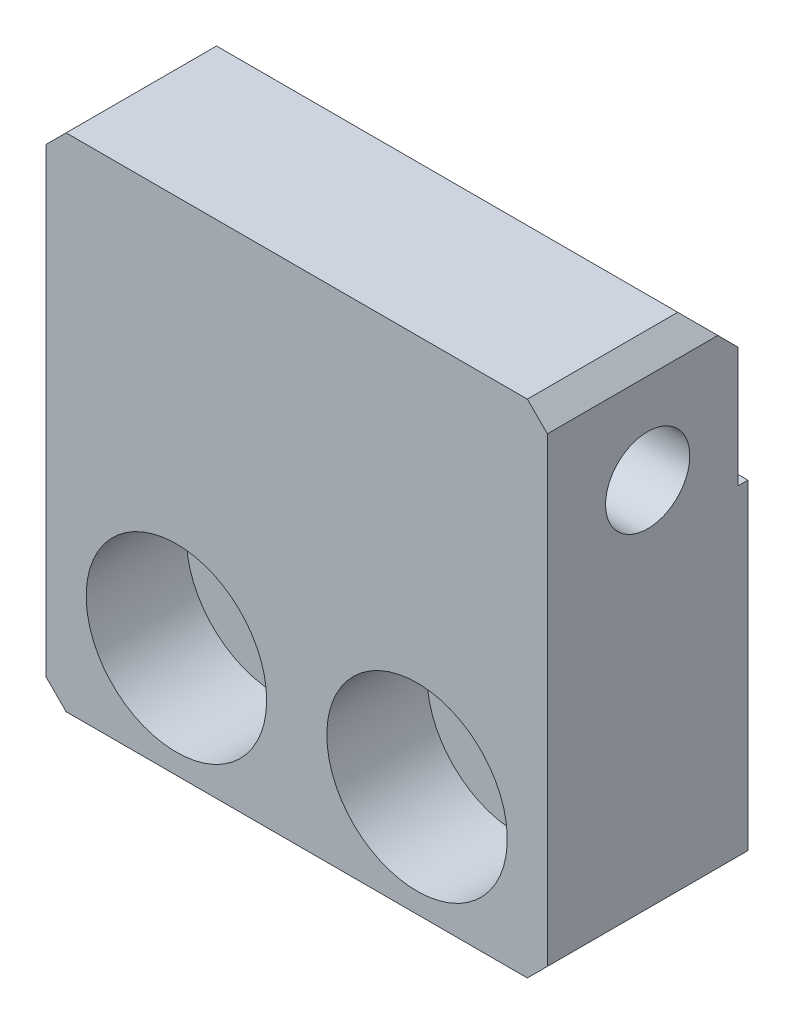
from build123d import *

# Parameters (mm, degrees)
SKETCH1_W           = 25
SKETCH1_H           = 25
BOSS_EXTRUDE1_DEPTH = 10
SKETCH3_R           = 4.5
CUT_EXTRUDE2_DEPTH  = 5
SKETCH4_R           = 2.25
CUT_EXTRUDE3_DEPTH  = 14
SKETCH5_R           = 0.905939467
CUT_EXTRUDE4_DEPTH  = 31
M5_TAPPED_HOLE1_D   = 4.2
CHAMFER1_SIZE       = 1
SKETCH8_W           = 0.5
SKETCH8_H           = 8
CUT_EXTRUDE5_DEPTH  = 31
CHAMFER2_SIZE       = 2


with BuildPart() as part:
    # Sketch1 → Boss-Extrude1 (new body)
    with BuildSketch(Plane.XY):
        Rectangle(SKETCH1_W, SKETCH1_H)
    extrude(amount=BOSS_EXTRUDE1_DEPTH)

    # Sketch3 → Cut-Extrude2 (cut)
    with BuildSketch(Plane.XY.offset(10)):
        with Locations((-6, -7)):
            Circle(SKETCH3_R)
        with Locations(Location((6, -7, 0), (0, 0, 180))):
            Circle(SKETCH3_R)
    extrude(amount=-CUT_EXTRUDE2_DEPTH, mode=Mode.SUBTRACT)

    # Sketch4 → Cut-Extrude3 (cut)
    with BuildSketch(Plane.XY.offset(10)):
        with Locations((-6, -7)):
            Circle(SKETCH4_R)
        with Locations((6, -7)):
            Circle(SKETCH4_R)
    extrude(amount=-CUT_EXTRUDE3_DEPTH, mode=Mode.SUBTRACT)

    # Sketch5 → Cut-Extrude4 (cut)
    with BuildSketch(Plane.ZY.offset(12.5)):
        with Locations(Location((5, 7, 0), (0, 0, 270))):
            Circle(SKETCH5_R)
    extrude(amount=-CUT_EXTRUDE4_DEPTH, mode=Mode.SUBTRACT)

    # M5 Tapped Hole1 (through all)
    with Locations(Plane(origin=(-12.5, 7, 5), x_dir=(0, -1, 0), z_dir=(-1, 0, 0))):
        with Locations((0, 0)):
            Hole(M5_TAPPED_HOLE1_D / 2)

    # Chamfer1
    chamfer1_edges = [part.edges().sort_by_distance(p)[0] for p in [
        (12.5, -12.5, 5),
        (-12.5, -12.5, 5),
        (-12.5, 12.5, 5),
        (12.5, 12.5, 5),
    ]]
    chamfer(chamfer1_edges, length=CHAMFER1_SIZE)

    # Sketch8 → Cut-Extrude5 (cut)
    with BuildSketch(Plane.ZY.offset(12.5)):
        with Locations((0.25, 8.5)):
            Rectangle(SKETCH8_W, SKETCH8_H)
    extrude(amount=-CUT_EXTRUDE5_DEPTH, mode=Mode.SUBTRACT)

    # Chamfer2
    chamfer2_edges = [part.edges().sort_by_distance(p)[0] for p in [
        (0, 12.5, 0.5),
    ]]
    chamfer(chamfer2_edges, length=CHAMFER2_SIZE)


solid = part.part
